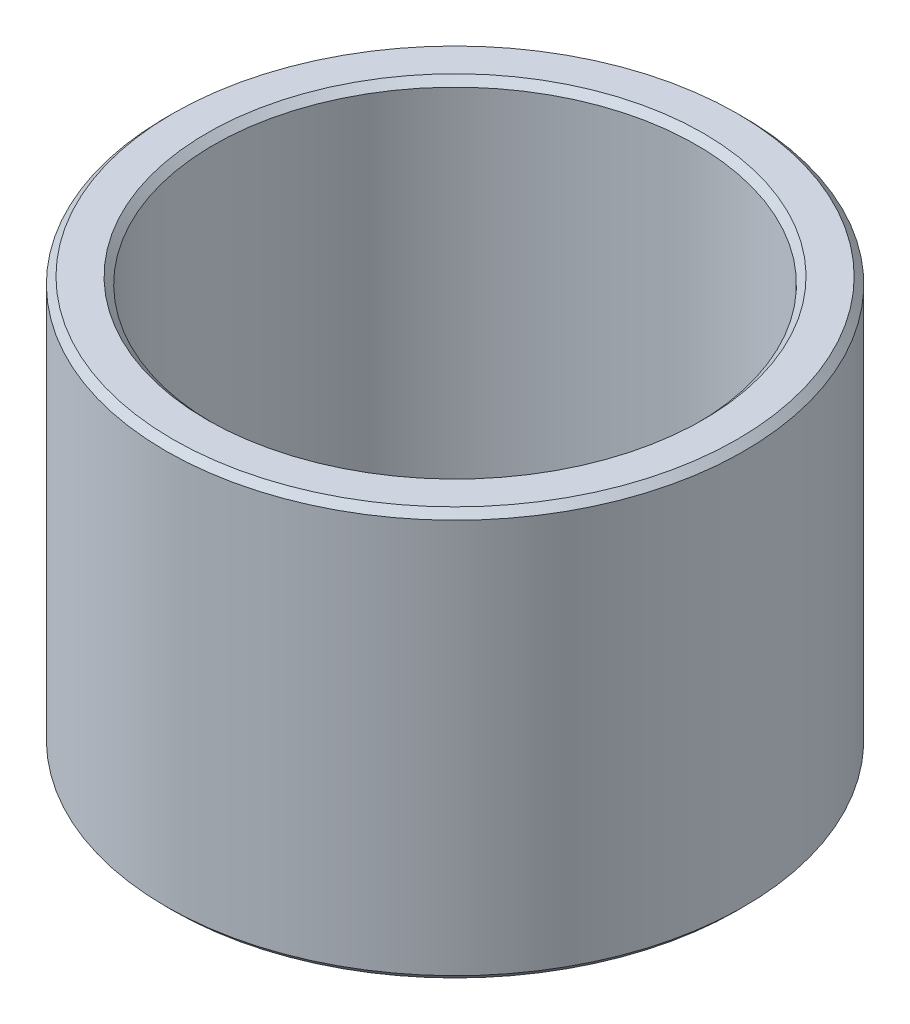
from build123d import *

# Parameters (mm, degrees)
SKETCH1_R           = 42.5
SKETCH1_R_2         = 35.5
BOSS_EXTRUDE1_DEPTH = 60
CHAMFER2_SIZE       = 1


with BuildPart() as part:
    # Sketch1 → Boss-Extrude1 (new body)
    with BuildSketch(Plane(origin=(0, 0, 0), x_dir=(1, 0, 0), z_dir=(0, 1, 0))):
        with Locations(Location((0, 0, 0), (0, 0, 270))):
            Circle(SKETCH1_R)
        with Locations(Location((0, 0, 0), (0, 0, 270))):
            Circle(SKETCH1_R_2, mode=Mode.SUBTRACT)
    extrude(amount=BOSS_EXTRUDE1_DEPTH)

    # Chamfer2
    chamfer2_edges = [part.edges().sort_by_distance(p)[0] for p in [
        (0, 0, -42.5),
        (0, 60, -42.5),
        (0, 0, -35.5),
        (0, 60, -35.5),
    ]]
    chamfer(chamfer2_edges, length=CHAMFER2_SIZE)


solid = part.part
